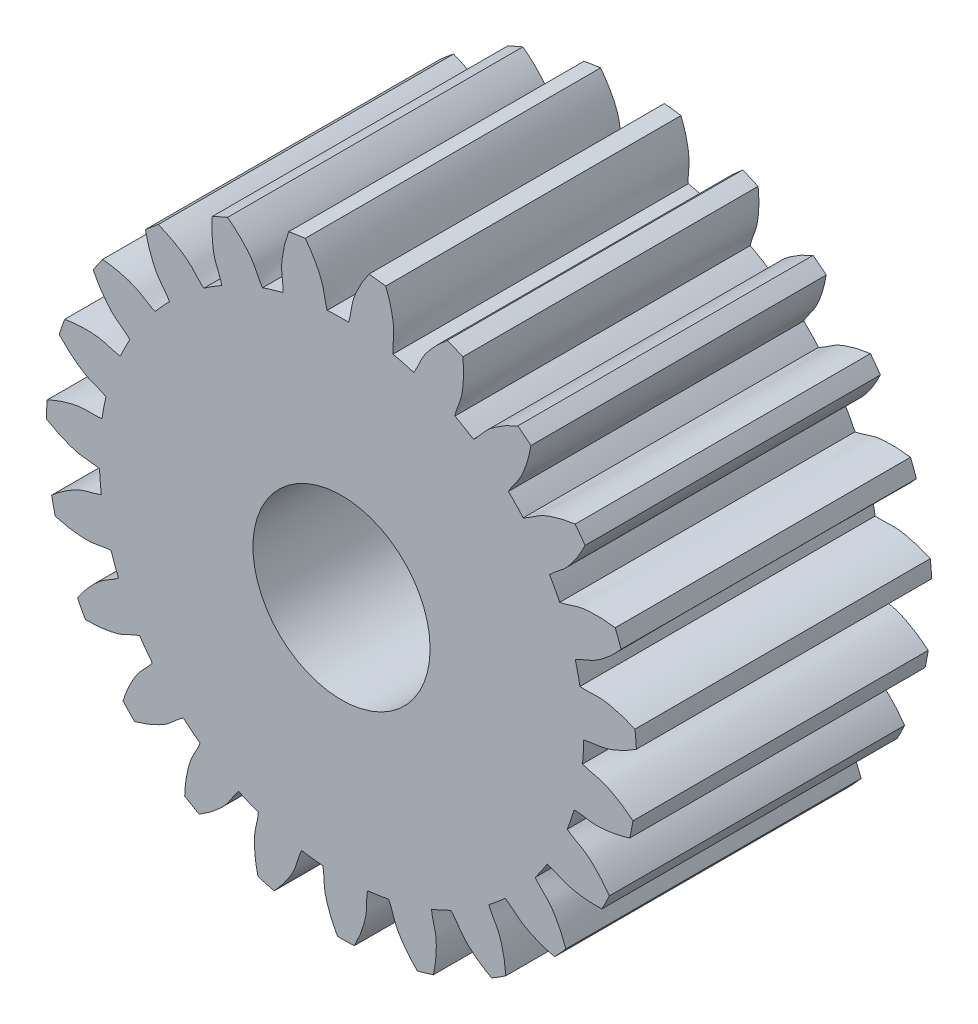
SolidWorks part; units mm, degrees
ref_plane "Front Plane" through (0, 0, 0) normal (0, 0, 1) x (1, 0, 0)
ref_plane "Top Plane" through (0, 0, 0) normal (0, 1, 0) x (1, 0, 0)
ref_plane "Right Plane" through (0, 0, 0) normal (1, 0, 0) x (0, 0, -1)
sketch "Sketch1" plane through (0, 0, 0) normal (0, 0, 1) x (1, 0, 0)
  circle A0 centre (0, 0) radius 123
extrude "Boss-Extrude1" add sketch "Sketch1" along normal blind 150
sketch "Sketch2" plane through (0, 0, 0) normal (0, 0, 1) x (1, 0, 0)
  arc A0 (149.0662, 16.711) -> (149.7751, 8.2101) centre (0, 0) cw
  arc A1 (121.1079, 21.4913) -> (122.9948, -1.135) centre (0, 0) cw
  spline S0 degree 3 poles (149.7751, 8.2101) (147.2262, 6.5422) (143.3086, 4.2723) (137.8542, 1.9501) (131.6634, -0.1567) (126.4899, -0.1416) (122.9948, -1.135) knots 0 0 0 0 0.318898 0.471672 0.619977 1 1 1 1
  spline S1 degree 3 poles (149.0662, 16.711) (146.2763, 17.9337) (142.0367, 19.5233) (136.2731, 20.9101) (129.8188, 21.9623) (124.7193, 21.0905) (121.1079, 21.4913) knots 0 0 0 0 0.318898 0.471672 0.619977 1 1 1 1
extrude "Boss-Extrude2" add sketch "Sketch2" along normal blind 150
pattern_circular "CirPattern1" count 23 over 360 about axis through (0, 0, 150) along (0, 0, -1) of "Boss-Extrude2"
sketch "Sketch3" plane through (0, 0, 150) normal (0, 0, 1) x (1, 0, 0)
  circle A0 centre (0, 0) radius 138 construction
  dimension "D1" = 276
sketch "Sketch4" plane through (0, 0, 0) normal (0, 1, 0) x (1, 0, 0)
  line L0 (0, 7.9852) -> (0, -156.706) construction
  line L1 (0, -150) -> (0, 0) construction
sketch "Sketch5" plane through (0, 0, 150) normal (0, 0, 1) x (1, 0, 0)
  circle A0 centre (0, 0) radius 45
extrude "Cut-Extrude1" cut sketch "Sketch5" against normal up to next
sketch "Sketch6" plane through (0, 0, 150) normal (0, 0, 1) x (1, 0, 0)
  circle A0 centre (0, 0) radius 132.5
  dimension "D1" = 265
